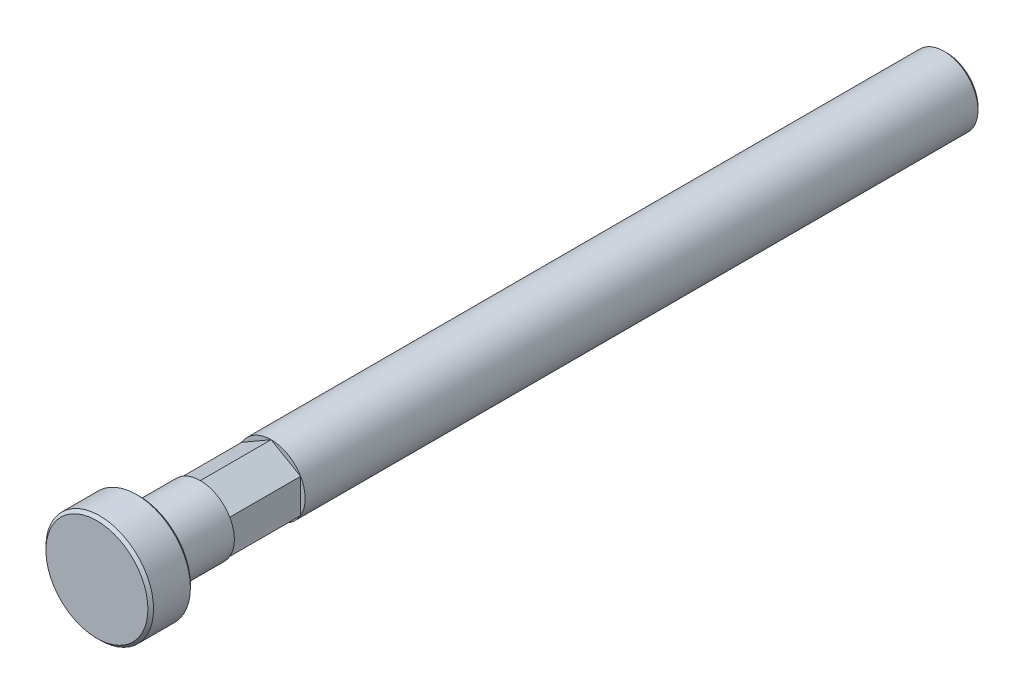
from build123d import *

# Parameters (mm, degrees)
BOSS_EXTRUDE1_DEPTH = 50
SKETCH2_R           = 24
BOSS_EXTRUDE2_DEPTH = 43
SKETCH3_R           = 38
BOSS_EXTRUDE3_DEPTH = 30
BOSS_EXTRUDE4_START = 477
SKETCH4_R           = 24
BOSS_EXTRUDE4_DEPTH = 477
CHAMFER1_SIZE       = 2


with BuildPart() as part:
    # Sketch1 → Boss-Extrude1 (new body)
    with BuildSketch(Plane.XY):
        Polygon((20.784609691, 12), (0, 24), (-20.784609691, 12), (-20.784609691, -12), (0, -24), (20.784609691, -12), align=None)
    extrude(amount=BOSS_EXTRUDE1_DEPTH)

    # Sketch2 → Boss-Extrude2 (add)
    with BuildSketch(Plane.XY.offset(50)):
        with Locations(Location((0, 0, 0), (0, 0, 150))):
            Circle(SKETCH2_R)
    extrude(amount=BOSS_EXTRUDE2_DEPTH)

    # Sketch3 → Boss-Extrude3 (add)
    with BuildSketch(Plane.XY.offset(93)):
        Circle(SKETCH3_R)
    extrude(amount=BOSS_EXTRUDE3_DEPTH)

    # Sketch4 → Boss-Extrude4 (add)
    with BuildSketch(Plane(origin=(0, 0, 0), x_dir=(-1, 0, 0), z_dir=(0, 0, -1)).offset(BOSS_EXTRUDE4_START)):
        with Locations(Location((0, 0, 0), (0, 0, 30))):
            Circle(SKETCH4_R)
    extrude(amount=-BOSS_EXTRUDE4_DEPTH)

    # Chamfer1
    chamfer1_edges = [part.edges().sort_by_distance(p)[0] for p in [
        (-38, 0, 93),
        (-38, 0, 123),
        (20.784609691, -12, -477),
    ]]
    chamfer(chamfer1_edges, length=CHAMFER1_SIZE)


solid = part.part
